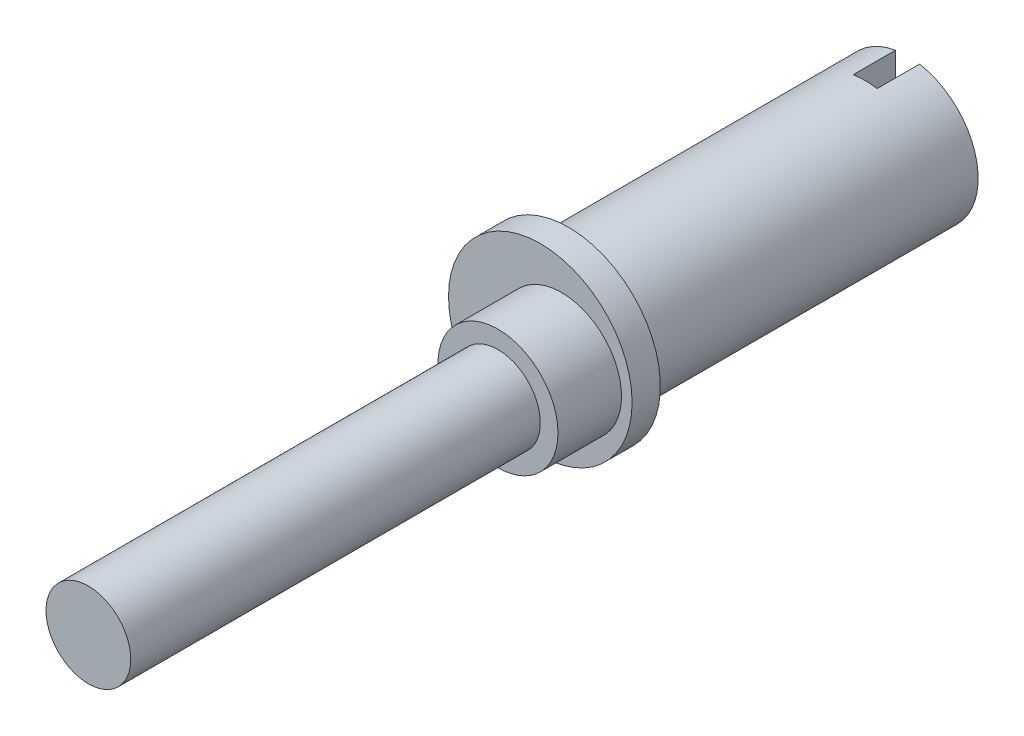
from build123d import *

# Parameters (mm, degrees)
SKETCH1_R           = 5
BOSS_EXTRUDE1_DEPTH = 25
SKETCH2_R           = 6.5
BOSS_EXTRUDE2_DEPTH = 1
SKETCH3_R           = 4.25
BOSS_EXTRUDE3_DEPTH = 4.5
SKETCH4_R           = 3
BOSS_EXTRUDE4_DEPTH = 29
SKETCH6_W           = 1.7
SKETCH6_H           = 11.931395552
CUT_EXTRUDE1_DEPTH  = 3
BOSS_EXTRUDE5_START = 1
SKETCH7_R           = 6.5
BOSS_EXTRUDE5_DEPTH = 1


with BuildPart() as part:
    # Sketch1 → Boss-Extrude1 (new body)
    with BuildSketch(Plane.XY):
        Circle(SKETCH1_R)
    extrude(amount=BOSS_EXTRUDE1_DEPTH)

    # Sketch2 → Boss-Extrude2 (add)
    with BuildSketch(Plane.XY.offset(25)):
        Circle(SKETCH2_R)
    extrude(amount=BOSS_EXTRUDE2_DEPTH)

    # Sketch3 → Boss-Extrude3 (add)
    with BuildSketch(Plane.XY.offset(26)):
        with Locations((1.5, 0)):
            Circle(SKETCH3_R)
    extrude(amount=BOSS_EXTRUDE3_DEPTH)

    # Sketch4 → Boss-Extrude4 (add)
    with BuildSketch(Plane.XY.offset(30.5)):
        with Locations(Location((1.5, 0, 0), (0, 0, 180))):
            Circle(SKETCH4_R)
    extrude(amount=BOSS_EXTRUDE4_DEPTH)

    # Sketch6 → Cut-Extrude1 (cut)
    with BuildSketch(Plane(origin=(0, 0, 0), x_dir=(-1, 0, 0), z_dir=(0, 0, -1))):
        Rectangle(SKETCH6_W, SKETCH6_H)
    extrude(amount=-CUT_EXTRUDE1_DEPTH, mode=Mode.SUBTRACT)

    # Sketch7 → Boss-Extrude5 (add)
    with BuildSketch(Plane(origin=(0, 0, 25), x_dir=(-1, 0, 0), z_dir=(0, 0, -1)).offset(BOSS_EXTRUDE5_START)):
        Circle(SKETCH7_R)
    extrude(amount=-BOSS_EXTRUDE5_DEPTH)


solid = part.part
